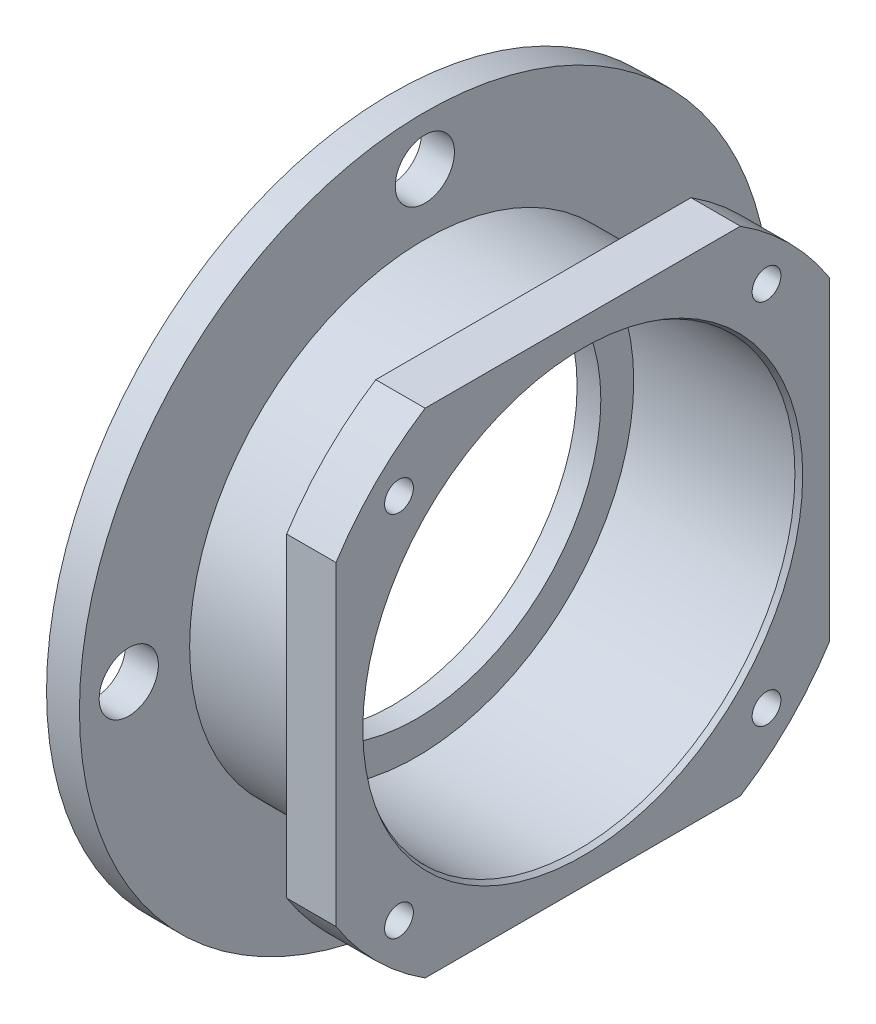
from build123d import *

# Parameters (mm, degrees)
SKETCH5_R          = 152.5
SKETCH5_R_2        = 141.5
CUT_EXTRUDE1_DEPTH = 5.9
SKETCH6_R          = 135
SKETCH6_R_2        = 124
CUT_EXTRUDE2_DEPTH = 5.9
SKETCH7_R          = 18
CUT_EXTRUDE3_DEPTH = 20
CIRPATTERN1_COUNT  = 4
CIRPATTERN2_COUNT  = 4
CUT_EXTRUDE4_DEPTH = 30
CHAMFER1_SIZE      = 3
CHAMFER1_SIZE2     = 1.732050808
CHAMFER2_SIZE      = 1
CHAMFER2_SIZE2     = 0.577350269


with BuildPart() as part:
    # Sketch4 → Revolve1 (revolve)
    with BuildSketch(Plane.XY, mode=Mode.PRIVATE) as revolve1_sk:
        Polygon((-62.794117647, 112), (-62.794117647, 210), (-42.794117647, 210), (-42.794117647, 143), (23.205882353, 143), (23.205882353, 178), (53.205882353, 178), (53.205882353, 132), (-47.794117647, 132), (-47.794117647, 112), align=None)
    revolve(revolve1_sk.sketch.rotate(Axis((-131.764705882, 0, 0), (1, 0, 0)), 90), axis=Axis((-131.764705882, 0, 0), (1, 0, 0)))

    # Sketch5 → Cut-Extrude1 (cut)
    with BuildSketch(Plane.ZY.offset(62.794117647)):
        Circle(SKETCH5_R)
        Circle(SKETCH5_R_2, mode=Mode.SUBTRACT)
    extrude(amount=-CUT_EXTRUDE1_DEPTH, mode=Mode.SUBTRACT)

    # Sketch6 → Cut-Extrude2 (cut)
    with BuildSketch(Plane.ZY.offset(62.794117647)):
        Circle(SKETCH6_R)
        Circle(SKETCH6_R_2, mode=Mode.SUBTRACT)
    extrude(amount=-CUT_EXTRUDE2_DEPTH, mode=Mode.SUBTRACT)

    # Sketch7 → Cut-Extrude3 (cut)
    with BuildSketch(Plane.ZY.offset(62.794117647)):
        with Locations((0, 180)):
            Circle(SKETCH7_R)
    cut_extrude3 = extrude(amount=-CUT_EXTRUDE3_DEPTH, mode=Mode.SUBTRACT)

    # CirPattern1: Cut-Extrude3 ×4 about axis
    cirpattern1_axis = Axis((0, 0, 0), (1, 0, 0))
    for i in range(1, CIRPATTERN1_COUNT):
        add(cut_extrude3.rotate(cirpattern1_axis, i * 360 / CIRPATTERN1_COUNT), mode=Mode.SUBTRACT)

    # Sketch9 → M20 Tapped Hole1 (revolve, cut)
    with BuildSketch(Plane(origin=(53.205882353, 111.722871427, -111.722871427), x_dir=(0, 0, -1), z_dir=(0, 1, 0))):
        Polygon((0, 0), (0, 57.757530416), (8.75, 52.5), (8.75, 0), align=None)
    m20_tapped_hole1 = revolve(axis=Axis((59.555882353, 111.722871427, -111.722871427), (-1, 0, 0)), mode=Mode.SUBTRACT)

    # CirPattern2: M20 Tapped Hole1 ×4 about axis
    cirpattern2_axis = Axis((0, 0, 0), (1, 0, 0))
    for i in range(1, CIRPATTERN2_COUNT):
        add(m20_tapped_hole1.rotate(cirpattern2_axis, i * 360 / CIRPATTERN2_COUNT), mode=Mode.SUBTRACT)

    # Sketch12 → Cut-Extrude4 (cut)
    with BuildSketch(Plane(origin=(53.205882353, 0, 0), x_dir=(0, 0, -1), z_dir=(1, 0, 0))):
        with BuildLine():
            Line((-95.833188406, 150), (95.833188406, 150))
            ThreePointArc((95.833188406, 150), (0, 178), (-95.833188406, 150))
        make_face()
        with BuildLine():
            Line((-150, 95.833188406), (-150, -95.833188406))
            ThreePointArc((-150, -95.833188406), (-178, 0), (-150, 95.833188406))
        make_face()
        with BuildLine():
            Line((-95.833188406, -150), (95.833188406, -150))
            ThreePointArc((95.833188406, -150), (0, -178), (-95.833188406, -150))
        make_face()
        with BuildLine():
            Line((150, 95.833188406), (150, -95.833188406))
            ThreePointArc((150, -95.833188406), (178, 0), (150, 95.833188406))
        make_face()
    extrude(amount=-CUT_EXTRUDE4_DEPTH, mode=Mode.SUBTRACT)

    # Chamfer1
    chamfer1_edges = [part.edges().sort_by_distance(p)[0] for p in [
        (53.205882353, 0, -132),
    ]]
    chamfer1_side = [part.faces().sort_by_distance(p)[0] for p in [
        (2.705882353, 0, -132),
    ]]
    chamfer(chamfer1_edges, length=CHAMFER1_SIZE, length2=CHAMFER1_SIZE2, reference=chamfer1_side[0])

    # Chamfer2
    chamfer2_edges = [part.edges().sort_by_distance(p)[0] for p in [
        (-62.794117647, 0, -112),
    ]]
    chamfer2_side = [part.faces().sort_by_distance(p)[0] for p in [
        (-62.794117647, 0, -120.492750365),
    ]]
    chamfer(chamfer2_edges, length=CHAMFER2_SIZE, length2=CHAMFER2_SIZE2, reference=chamfer2_side[0])


solid = part.part
